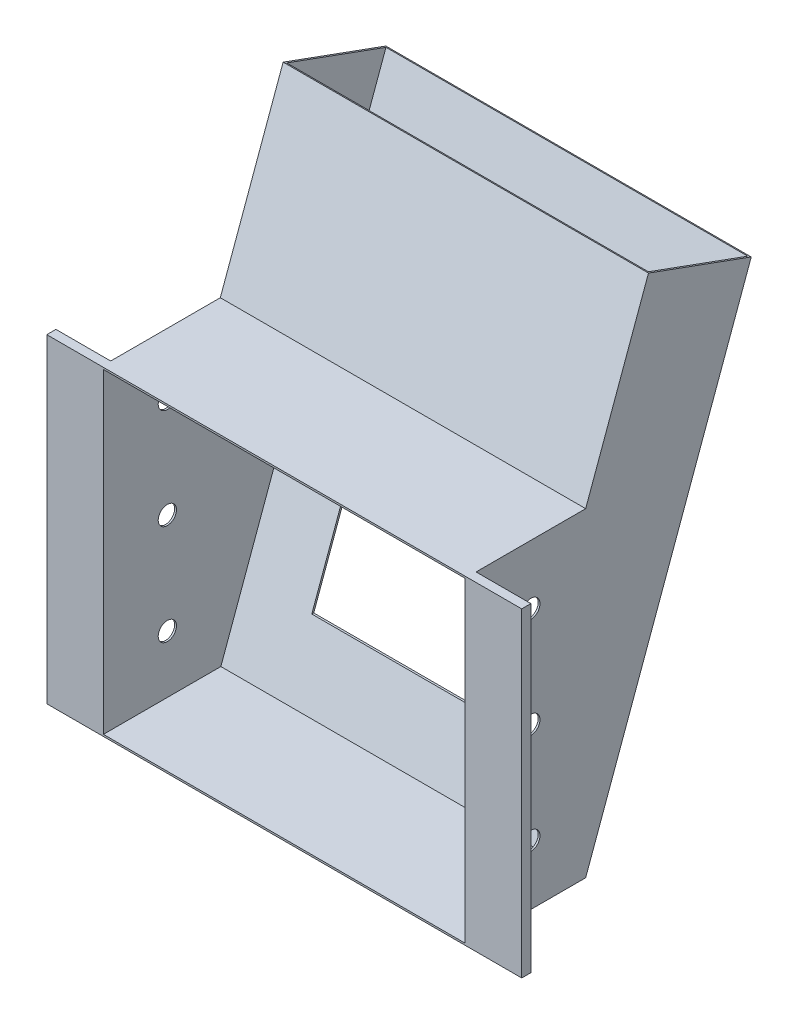
SolidWorks part; units mm, degrees
ref_plane "前视基准面" through (0, 0, 0) normal (0, 0, 1) x (1, 0, 0)
ref_plane "上视基准面" through (0, 0, 0) normal (0, 1, 0) x (1, 0, 0)
ref_plane "右视基准面" through (0, 0, 0) normal (1, 0, 0) x (0, 0, -1)
sketch "草图1" plane through (0, 0, 0) normal (0, 0, 1) x (1, 0, 0)
  line L1 (-200, -175) -> (200, -175)
  line L2 (-200, -175) -> (-200, 175)
  line L3 (-200, 175) -> (200, 175)
  line L4 (200, -175) -> (200, 175)
  line L5 (-200, -175) -> (200, 175) construction
  line L6 (-200, 175) -> (200, -175) construction
  point P0 (0, 0)
  dimension "D1" = 400
  dimension "D2" = 350
extrude "凸台-拉伸1" add sketch "草图1" along normal blind 130
sketch "草图7" plane through (-200, 0, 0) normal (-1, 0, 0) x (0, 0, 1)
  line L0 (0, 175) -> (-68.7828, 363.9793)
  line L1 (-68.7828, 363.9793) -> (-181.2707, 323.0371)
  line L2 (-181.2707, 323.0371) -> (0, -175)
  line L3 (0, -175) -> (0, 175)
  line L4 (130, 175) -> (0, 175) construction
  dimension "D1" = 110
  dimension "D2" = 530
extrude "凸台-拉伸5" add sketch "草图7" against normal up to surface (400 mm away) up to face at (200, 0, 65)
shell "抽壳2" thickness 2
sketch "草图3" plane through (0, 0, 130) normal (0, 0, 1) x (1, 0, 0)
  line L0 (-200, -175) -> (200, -175) construction
  line L1 (-200, 175) -> (-260, 175)
  line L2 (-200, 175) -> (-200, -175)
  line L3 (-200, -175) -> (-260, -175)
  line L4 (-260, 175) -> (-260, -175)
  line L6 (200, 175) -> (260, 175)
  line L7 (200, 175) -> (200, -175)
  line L8 (200, -175) -> (260, -175)
  line L9 (260, 175) -> (260, -175)
  dimension "D1" = 60
extrude "凸台-拉伸2" add sketch "草图3" against normal blind 10
sketch "草图8" plane through (0, 0, 130) normal (0, 0, 1) x (1, 0, 0)
  line L0 (0, 175) -> (0, -173) construction
  line L1 (260, 175) -> (-260, 175) construction
  line L2 (-198, -173) -> (198, -173) construction
  line L4 (-125, -100) -> (125, -100)
  line L5 (-125, -100) -> (-125, 100)
  line L6 (-125, 100) -> (125, 100)
  line L7 (125, -100) -> (125, 100)
  line L8 (-125, -100) -> (125, 100) construction
  line L9 (-125, 100) -> (125, -100) construction
  point P6 (0, 0)
  dimension "D1" = 250
  dimension "D2" = 200
extrude "切除-拉伸1" cut sketch "草图8" against normal through all
sketch "草图9" plane through (200, 0, 0) normal (1, 0, 0) x (0, 0, -1)
  line L0 (-120, -175) -> (0, -175) construction
  line L1 (-130, -175) -> (-130, 175) construction
  circle A0 centre (-60, 110) radius 10
  circle A1 centre (-60, -110) radius 10
  circle A2 centre (-60, 0) radius 10
  dimension "D1" = 20
  dimension "D2" = 220
  dimension "D3" = 65
  dimension "D4" = 70
  dimension "D5" = 110
extrude "切除-拉伸2" cut sketch "草图9" against normal through all
